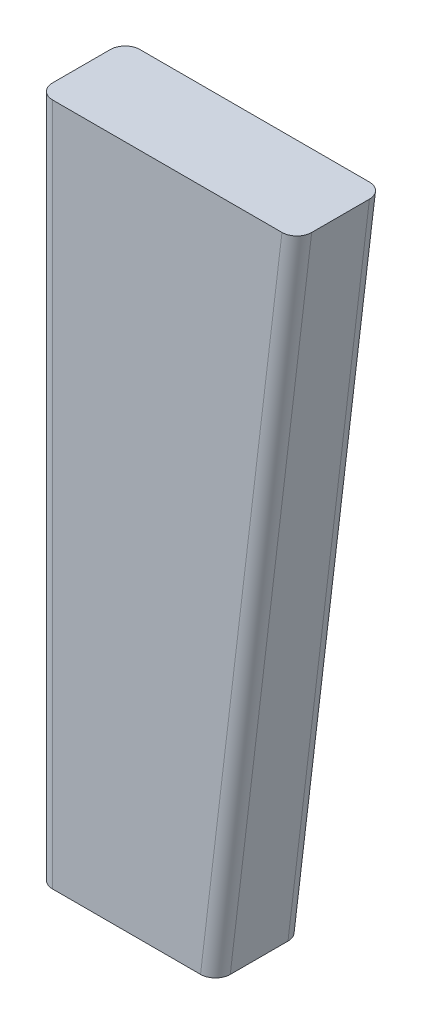
SolidWorks part; units mm, degrees
ref_plane "Front Plane" through (0, 0, 0) normal (0, 0, 1) x (1, 0, 0)
ref_plane "Top Plane" through (0, 0, 0) normal (0, 1, 0) x (1, 0, 0)
ref_plane "Right Plane" through (0, 0, 0) normal (1, 0, 0) x (0, 0, -1)
other "Configuration Table"
sketch "Sketch1" plane through (0, 0, 0) normal (0, 0, 1) x (1, 0, 0)
  line L0 (0, 0) -> (240, 0)
  line L1 (240, 0) -> (350, 923)
  line L2 (350, 923) -> (0, 923)
  line L3 (0, 923) -> (0, 0)
  dimension "D1" = 923
  dimension "D2" = 350
  dimension "D3" = 240
extrude "Boss-Extrude1" add sketch "Sketch1" along normal blind 118
fillet "Fillet1" radius 20 4 edges at (0, 461.5, 0) (0, 461.5, 118) (295, 461.5, 0) (295, 461.5, 118)
